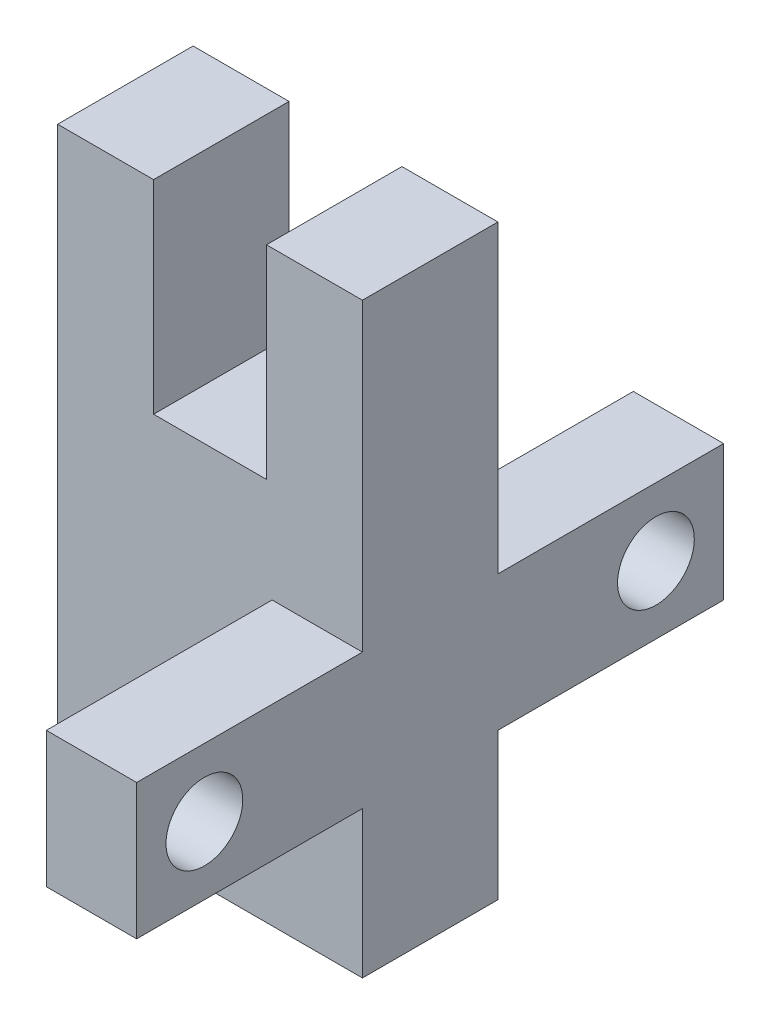
from build123d import *

# Parameters (mm, degrees)
BOSS_EXTRUDE1_DEPTH = 3
SKETCH2_W           = 26
SKETCH2_H           = 6
SKETCH2_R           = 1.7
BOSS_EXTRUDE2_DEPTH = 4


with BuildPart() as part:
    # Sketch1 → Boss-Extrude1 (new, symmetric)
    with BuildSketch(Plane.XY):
        Polygon((9.25, 0), (13.5, 0), (13.5, -26), (0, -26), (0, 0), (4.25, 0), (4.25, -9), (9.25, -9), align=None)
    extrude(amount=BOSS_EXTRUDE1_DEPTH, both=True)

    # Sketch2 → Boss-Extrude2 (add)
    with BuildSketch(Plane(origin=(13.5, 0, 0), x_dir=(0, 0, -1), z_dir=(1, 0, 0))):
        with Locations((0, -16.5)):
            Rectangle(SKETCH2_W, SKETCH2_H)
        with Locations(Location((-10, -16.5, 0), (0, 0, 90))):
            Circle(SKETCH2_R, mode=Mode.SUBTRACT)
        with Locations(Location((10, -16.5, 0), (0, 0, 90))):
            Circle(SKETCH2_R, mode=Mode.SUBTRACT)
    extrude(amount=-BOSS_EXTRUDE2_DEPTH)


solid = part.part
